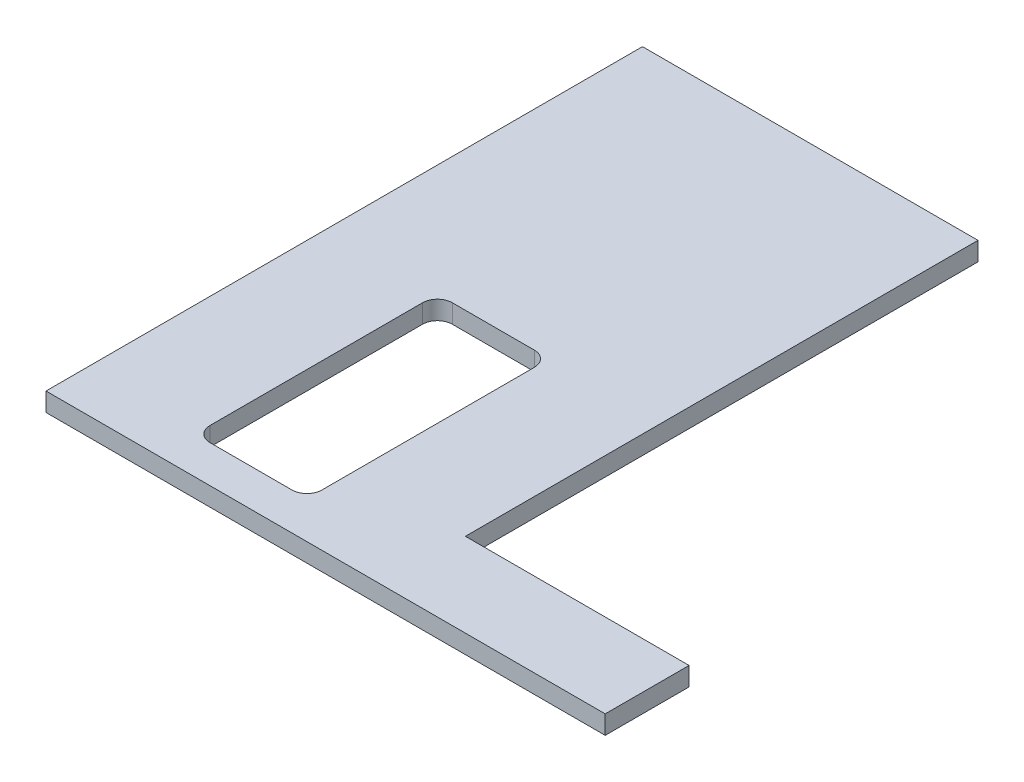
SolidWorks part; units mm, degrees
ref_plane "Front Plane" through (0, 0, 0) normal (0, 0, 1) x (1, 0, 0)
ref_plane "Top Plane" through (0, 0, 0) normal (0, 1, 0) x (1, 0, 0)
ref_plane "Right Plane" through (0, 0, 0) normal (1, 0, 0) x (0, 0, -1)
sketch "Sketch1" plane through (0, 0, 0) normal (0, 1, 0) x (1, 0, 0)
  line L1 (-90, 160) -> (90, 160)
  line L2 (-90, 160) -> (-90, -160)
  line L3 (-90, -160) -> (90, -160)
  line L4 (90, 160) -> (90, -160)
  line L5 (-90, 160) -> (90, -160) construction
  line L6 (-90, -160) -> (90, 160) construction
  point P0 (0, 0)
  dimension "D1" = 180
  dimension "D2" = 320
extrude "Boss-Extrude1" add sketch "Sketch1" along normal blind 10
sketch "Sketch2" plane through (0, 10, 0) normal (0, 1, 0) x (1, 0, 0)
  line L0 (0, -10) -> (0, 160) construction
  line L1 (30, -10) -> (-30, -10)
  line L2 (30, -10) -> (30, -140)
  line L3 (30, -140) -> (-30, -140)
  line L4 (-30, -10) -> (-30, -140)
  line L5 (90, 160) -> (-90, 160) construction
  line L6 (-90, -160) -> (90, -160) construction
  dimension "D1" = 20
  dimension "D2" = 60
  dimension "D3" = 130
extrude "Cut-Extrude1" cut sketch "Sketch2" against normal through all
fillet "Fillet1" radius 8 4 edges at (30, 5, 140) (-30, 5, 140) (-30, 5, 10) (30, 5, 10)
sketch "Sketch3" plane through (90, 0, 0) normal (1, 0, 0) x (0, 0, -1)
  line L0 (-160, 0) -> (160, 0) construction
  line L1 (-160, 10) -> (-115, 10)
  line L2 (-160, 10) -> (-160, 0)
  line L3 (-160, 0) -> (-115, 0)
  line L4 (-115, 10) -> (-115, 0)
  dimension "D1" = 45
extrude "Boss-Extrude2" add sketch "Sketch3" along normal blind 120
